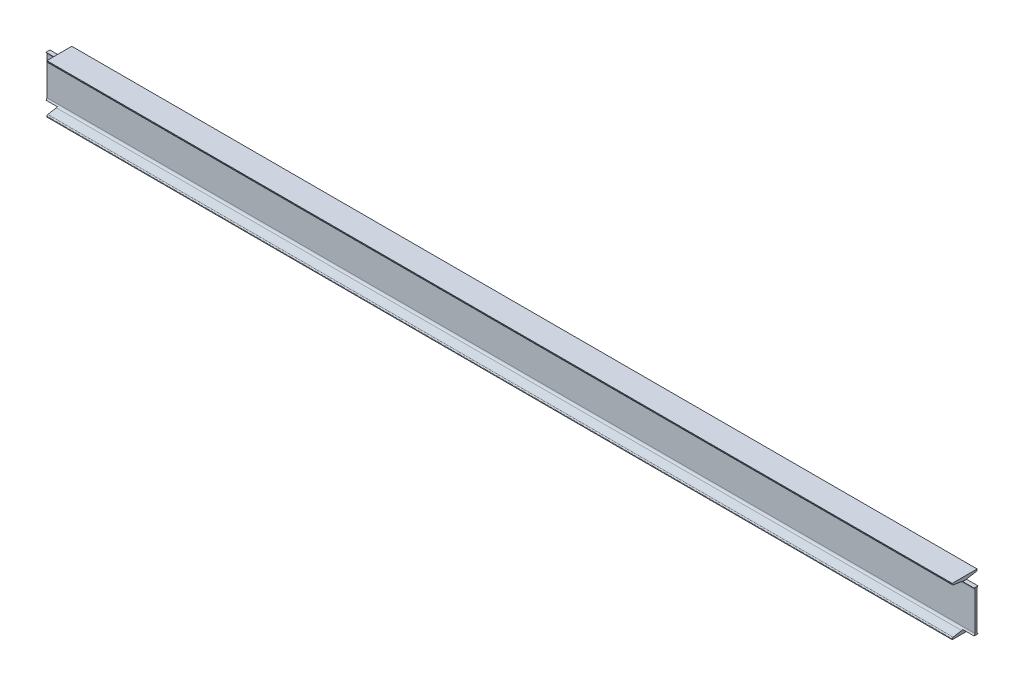
from build123d import *

# Parameters (mm, degrees)
BASE_DEPTH         = 3800
FILLET1_R          = 9
FILLET2_R          = 4.5
SKETCH_1_W         = 46.5
SKETCH_1_H         = 102
CUT_EXTRUDE1_DEPTH = 15
SKETCH2_W          = 46.5
SKETCH2_H          = 102
CUT_EXTRUDE2_DEPTH = 15


with BuildPart() as part:
    # Sketch1 → Base (new body)
    with BuildSketch(Plane(origin=(0, 0, 0), x_dir=(0, 0, -1), z_dir=(1, 0, 0))):
        Polygon((-51, 0), (51, 0), (51, 6.775), (4.5, 14.525), (4.5, 185.475), (51, 193.225), (51, 200), (-51, 200), (-51, 193.225), (-4.5, 185.475), (-4.5, 14.525), (-51, 6.775), align=None)
    extrude(amount=BASE_DEPTH)

    # Fillet1
    fillet1_edges = [part.edges().sort_by_distance(p)[0] for p in [
        (1900, 14.525, 4.5),
        (1900, 185.475, 4.5),
        (1900, 185.475, -4.5),
        (1900, 14.525, -4.5),
    ]]
    fillet(fillet1_edges, radius=FILLET1_R)

    # Fillet2
    fillet2_edges = [part.edges().sort_by_distance(p)[0] for p in [
        (1900, 6.775, 51),
        (1900, 193.225, 51),
        (1900, 193.225, -51),
        (1900, 6.775, -51),
    ]]
    fillet(fillet2_edges, radius=FILLET2_R)

    # 草图1 → Cut-Extrude1 (cut)
    with BuildSketch(Plane(origin=(0, 200, 0), x_dir=(1, 0, 0), z_dir=(0, 1, 0))):
        with Locations((23.25, 0)):
            Rectangle(SKETCH_1_W, SKETCH_1_H)
        with Locations((3776.75, 0)):
            Rectangle(SKETCH_1_W, SKETCH_1_H)
    extrude(amount=-CUT_EXTRUDE1_DEPTH, mode=Mode.SUBTRACT)

    # Sketch2 → Cut-Extrude2 (cut)
    with BuildSketch(Plane(origin=(0, 0, 0), x_dir=(-1, 0, 0), z_dir=(0, -1, 0))):
        with Locations((-23.25, 0)):
            Rectangle(SKETCH2_W, SKETCH2_H)
        with Locations((-3776.75, 0)):
            Rectangle(SKETCH2_W, SKETCH2_H)
    extrude(amount=-CUT_EXTRUDE2_DEPTH, mode=Mode.SUBTRACT)


solid = part.part
